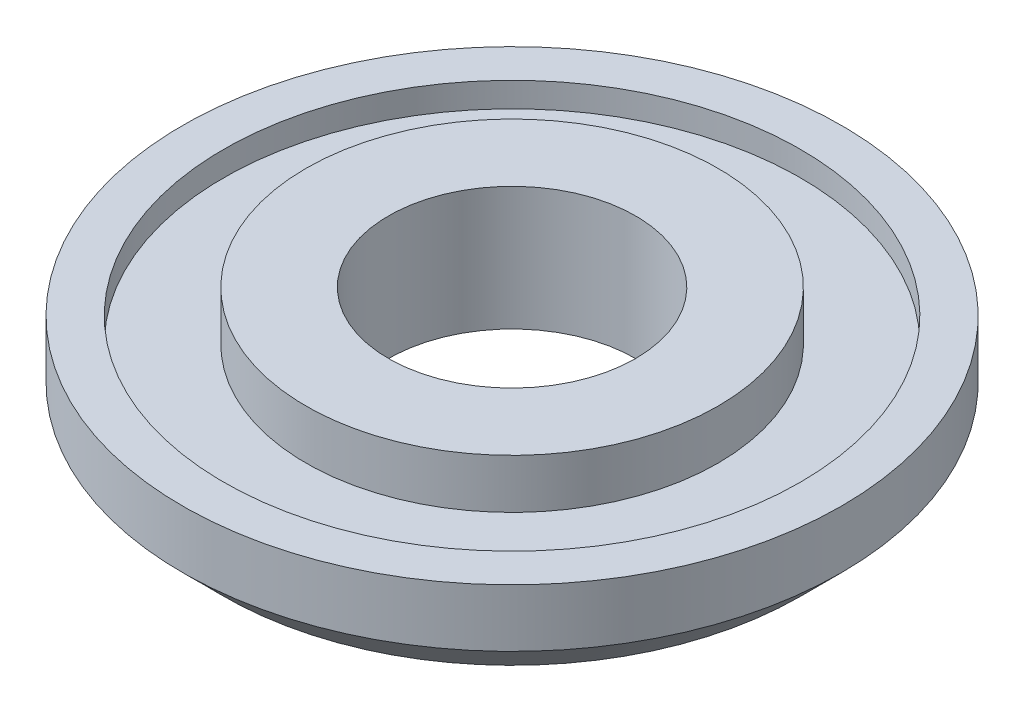
SolidWorks part; units mm, degrees
material "普通碳钢"
ref_plane "Front Plane" through (0, 0, 0) normal (0, 0, 1) x (1, 0, 0)
ref_plane "Top Plane" through (0, 0, 0) normal (0, 1, 0) x (1, 0, 0)
ref_plane "Right Plane" through (0, 0, 0) normal (1, 0, 0) x (0, 0, -1)
sketch "Sketch1" plane through (0, 0, 0) normal (0, 0, 1) x (1, 0, 0)
  line L0 (15, 517) -> (35, 517)
  line L2 (40, 522) -> (40, 529)
  line L3 (40, 529) -> (35, 529)
  line L4 (35, 529) -> (35, 526)
  line L5 (35, 526) -> (25, 526)
  line L6 (25, 526) -> (25, 532)
  line L7 (25, 532) -> (15, 532)
  line L8 (0, 517) -> (0, 561) construction
  line L9 (15, 532) -> (15, 517)
  line L13 (35, 517) -> (40, 522)
  point P1 (40, 517)
  dimension "D1" = 15
  dimension "D2" = 25
  dimension "D3" = 40
  dimension "D4" = 12
  dimension "D5" = 3
  dimension "D6" = 5
revolve "Revolve1" add sketch "Sketch1" angle 360 about L8
